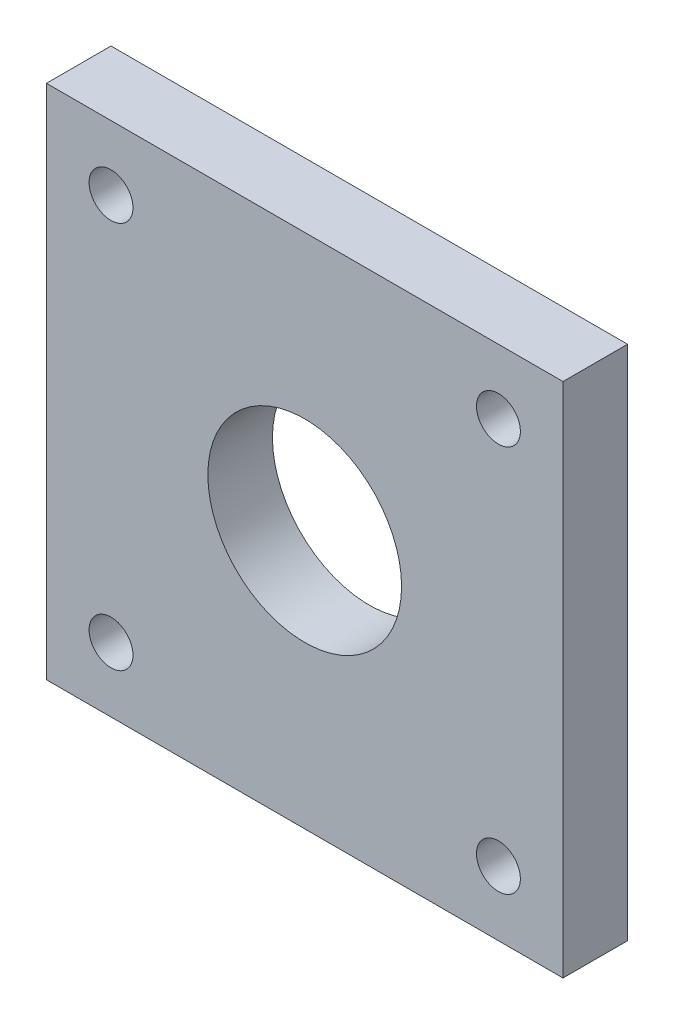
from build123d import *

# Parameters (mm, degrees)
SKETCH1_W             = 80
SKETCH1_H             = 80
BOSS_EXTRUDE1_DEPTH   = 10
M8_TAPPED_HOLE1_D     = 6.8
M8_TAPPED_HOLE1_DEPTH = 19.75
M8_TAPPED_HOLE1_TIP   = 2.042926105
SKETCH5_R             = 15
CUT_EXTRUDE1_DEPTH    = 10


with BuildPart() as part:
    # Sketch1 → Boss-Extrude1 (new body)
    with BuildSketch(Plane.XY):
        Rectangle(SKETCH1_W, SKETCH1_H)
    extrude(amount=BOSS_EXTRUDE1_DEPTH)

    # M8 Tapped Hole1
    with Locations(Plane.XY.offset(10)):
        with Locations((-30, 30), (30, 30), (30, -30), (-30, -30)):
            Hole(M8_TAPPED_HOLE1_D / 2, depth=M8_TAPPED_HOLE1_DEPTH)
            with Locations((0, 0, -(M8_TAPPED_HOLE1_DEPTH + M8_TAPPED_HOLE1_TIP / 2))):  # 118° drill point
                Cone(0, M8_TAPPED_HOLE1_D / 2, M8_TAPPED_HOLE1_TIP, mode=Mode.SUBTRACT)

    # Sketch5 → Cut-Extrude1 (cut)
    with BuildSketch(Plane.XY.offset(10)):
        Circle(SKETCH5_R)
    extrude(amount=-CUT_EXTRUDE1_DEPTH, mode=Mode.SUBTRACT)


solid = part.part
